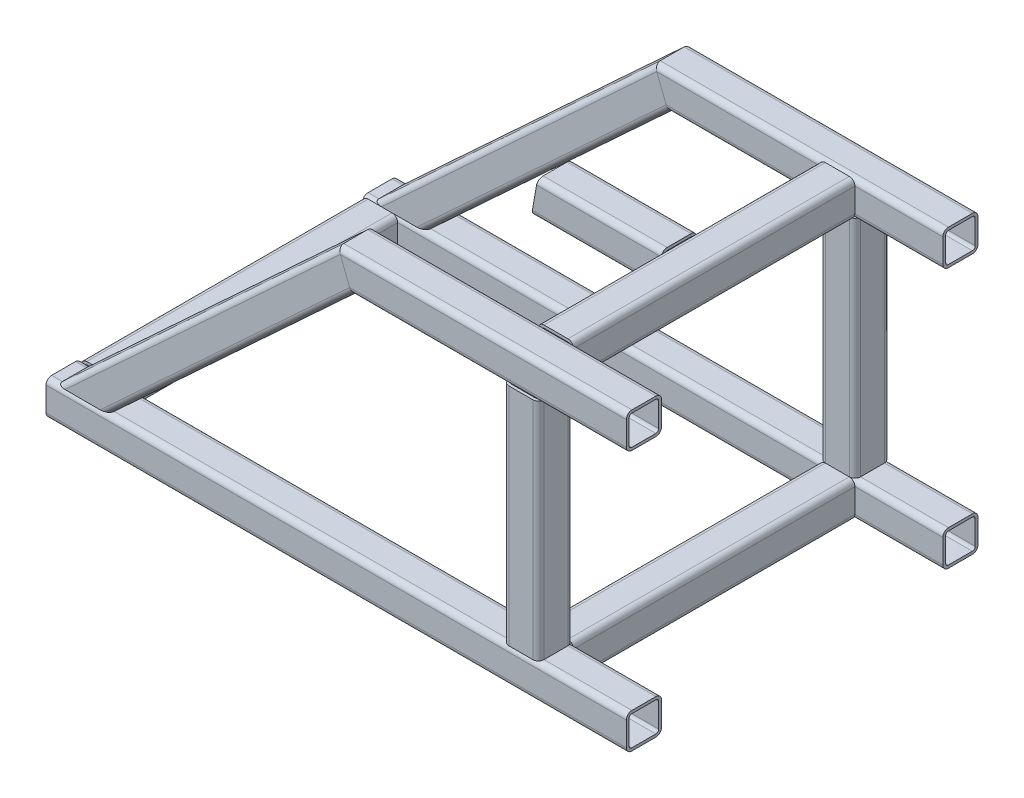
from build123d import *

# Parameters (mm, degrees)
GB_6728_1986_SQUARE_HOLLOW_SECTION_050_X_DEPTH = 400
GB_6728_1986_SQUARE_HOLLOW_SECTION_0_2_DEPTH   = 400
GB_6728_1986_SQUARE_HOLLOW_SECTION_0_3_DEPTH   = 825
GB_6728_1986_SQUARE_HOLLOW_SECTION_0_4_DEPTH   = 825
GB_6728_1986_SQUARE_HOLLOW_SECTION_0_5_DEPTH   = 211
GB_6728_1986_SQUARE_HOLLOW_SECTION_0_6_DEPTH   = 452
GB_6728_1986_SQUARE_HOLLOW_SECTION_0_8_DEPTH   = 372
GB_6728_1986_SQUARE_HOLLOW_SECTION_0_10_DEPTH  = 452
GB_6728_1986_SQUARE_HOLLOW_SECTION_0_13_DEPTH  = 372
GB_6728_1986_SQUARE_HOLLOW_SECTION_0_16_DEPTH  = 452
GB_6728_1986_SQUARE_HOLLOW_SECTION_0_19_DEPTH  = 544.885309033
GB_6728_1986_SQUARE_HOLLOW_SECTION_0_20_DEPTH  = 544.885309033
PART_RUN_ON_DEPTH                              = 409.789548
BODY_START                                     = 151.21090415
BODY_12_RUN_ON_DEPTH                           = 461.826729237
BODY_2_RUN_ON_DEPTH                            = 409.789548
BODY_11_RUN_ON_DEPTH                           = 461.826729237
CUT_EXTRUDE1_START                             = -50
CUT_EXTRUDE1_DEPTH                             = 50


with BuildPart() as part:
    # Sketch1 → Gb_6728-1986 square hollow section 050 X (new body)
    with BuildSketch(Plane(origin=(-250, 370, 450), x_dir=(0, 0, -1), z_dir=(1, 0, 0))):
        with BuildLine():
            Line((-17, -25), (17, -25))
            ThreePointArc((17, -25), (22.656854249, -22.656854249), (25, -17))
            Line((25, -17), (25, 17))
            ThreePointArc((25, 17), (22.656854249, 22.656854249), (17, 25))
            Line((17, 25), (-17, 25))
            ThreePointArc((-17, 25), (-22.656854249, 22.656854249), (-25, 17))
            Line((-25, 17), (-25, -17))
            ThreePointArc((-25, -17), (-22.656854249, -22.656854249), (-17, -25))
        make_face()
        with BuildLine():
            Line((-17, -21), (17, -21))
            ThreePointArc((17, -21), (19.828427125, -19.828427125), (21, -17))
            Line((21, -17), (21, 17))
            ThreePointArc((21, 17), (19.828427125, 19.828427125), (17, 21))
            Line((17, 21), (-17, 21))
            ThreePointArc((-17, 21), (-19.828427125, 19.828427125), (-21, 17))
            Line((-21, 17), (-21, -17))
            ThreePointArc((-21, -17), (-19.828427125, -19.828427125), (-17, -21))
        make_face(mode=Mode.SUBTRACT)
    extrude(amount=GB_6728_1986_SQUARE_HOLLOW_SECTION_050_X_DEPTH)

    # Sketch1 → part run on (add)
    with BuildSketch(Plane(origin=(-250, 370, 450), x_dir=(0, 0, -1), z_dir=(1, 0, 0))):
        with BuildLine():
            Line((-17, -25), (17, -25))
            ThreePointArc((17, -25), (22.656854249, -22.656854249), (25, -17))
            Line((25, -17), (25, 17))
            ThreePointArc((25, 17), (22.656854249, 22.656854249), (17, 25))
            Line((17, 25), (-17, 25))
            ThreePointArc((-17, 25), (-22.656854249, 22.656854249), (-25, 17))
            Line((-25, 17), (-25, -17))
            ThreePointArc((-25, -17), (-22.656854249, -22.656854249), (-17, -25))
        make_face()
        with BuildLine():
            Line((-17, -21), (17, -21))
            ThreePointArc((17, -21), (19.828427125, -19.828427125), (21, -17))
            Line((21, -17), (21, 17))
            ThreePointArc((21, 17), (19.828427125, 19.828427125), (17, 21))
            Line((17, 21), (-17, 21))
            ThreePointArc((-17, 21), (-19.828427125, 19.828427125), (-21, 17))
            Line((-21, 17), (-21, -17))
            ThreePointArc((-21, -17), (-19.828427125, -19.828427125), (-17, -21))
        make_face(mode=Mode.SUBTRACT)
    extrude(amount=-PART_RUN_ON_DEPTH)

    # Trim/Extend 3
    split(bisect_by=Plane(origin=(-250, 370, 450), x_dir=(-0.364623477, 0.931155046, 0), z_dir=(0.931155046, 0.364623477, 0)), keep=Keep.TOP)


with BuildPart() as body_2:
    # Sketch1 on segment 2 (carried to segment 2) → Gb_6728-1986 square hollow section 0 2 (new body)
    with BuildSketch(Plane(origin=(-250, 370, 0), x_dir=(0, 0, -1), z_dir=(1, 0, 0))):
        with BuildLine():
            Line((-17, -25), (17, -25))
            ThreePointArc((17, -25), (22.656854249, -22.656854249), (25, -17))
            Line((25, -17), (25, 17))
            ThreePointArc((25, 17), (22.656854249, 22.656854249), (17, 25))
            Line((17, 25), (-17, 25))
            ThreePointArc((-17, 25), (-22.656854249, 22.656854249), (-25, 17))
            Line((-25, 17), (-25, -17))
            ThreePointArc((-25, -17), (-22.656854249, -22.656854249), (-17, -25))
        make_face()
        with BuildLine():
            Line((-17, -21), (17, -21))
            ThreePointArc((17, -21), (19.828427125, -19.828427125), (21, -17))
            Line((21, -17), (21, 17))
            ThreePointArc((21, 17), (19.828427125, 19.828427125), (17, 21))
            Line((17, 21), (-17, 21))
            ThreePointArc((-17, 21), (-19.828427125, 19.828427125), (-21, 17))
            Line((-21, 17), (-21, -17))
            ThreePointArc((-21, -17), (-19.828427125, -19.828427125), (-17, -21))
        make_face(mode=Mode.SUBTRACT)
    extrude(amount=GB_6728_1986_SQUARE_HOLLOW_SECTION_0_2_DEPTH)

    # Sketch1 on segment 2 (carried to segment 2) → body 2 run on (add)
    with BuildSketch(Plane(origin=(-250, 370, 0), x_dir=(0, 0, -1), z_dir=(1, 0, 0))):
        with BuildLine():
            Line((-17, -25), (17, -25))
            ThreePointArc((17, -25), (22.656854249, -22.656854249), (25, -17))
            Line((25, -17), (25, 17))
            ThreePointArc((25, 17), (22.656854249, 22.656854249), (17, 25))
            Line((17, 25), (-17, 25))
            ThreePointArc((-17, 25), (-22.656854249, 22.656854249), (-25, 17))
            Line((-25, 17), (-25, -17))
            ThreePointArc((-25, -17), (-22.656854249, -22.656854249), (-17, -25))
        make_face()
        with BuildLine():
            Line((-17, -21), (17, -21))
            ThreePointArc((17, -21), (19.828427125, -19.828427125), (21, -17))
            Line((21, -17), (21, 17))
            ThreePointArc((21, 17), (19.828427125, 19.828427125), (17, 21))
            Line((17, 21), (-17, 21))
            ThreePointArc((-17, 21), (-19.828427125, 19.828427125), (-21, 17))
            Line((-21, 17), (-21, -17))
            ThreePointArc((-21, -17), (-19.828427125, -19.828427125), (-17, -21))
        make_face(mode=Mode.SUBTRACT)
    extrude(amount=-BODY_2_RUN_ON_DEPTH)

    # Trim/Extend 4
    split(bisect_by=Plane(origin=(-250, 370, 0), x_dir=(-0.364623477, 0.931155046, 0), z_dir=(0.931155046, 0.364623477, 0)), keep=Keep.TOP)


with BuildPart() as body_3:
    # Sketch1 on segment 3 (carried to segment 3) → Gb_6728-1986 square hollow section 0 3 (new body)
    with BuildSketch(Plane(origin=(-675, 0, 450), x_dir=(0, 0, -1), z_dir=(1, 0, 0))):
        with BuildLine():
            Line((-17, -25), (17, -25))
            ThreePointArc((17, -25), (22.656854249, -22.656854249), (25, -17))
            Line((25, -17), (25, 17))
            ThreePointArc((25, 17), (22.656854249, 22.656854249), (17, 25))
            Line((17, 25), (-17, 25))
            ThreePointArc((-17, 25), (-22.656854249, 22.656854249), (-25, 17))
            Line((-25, 17), (-25, -17))
            ThreePointArc((-25, -17), (-22.656854249, -22.656854249), (-17, -25))
        make_face()
        with BuildLine():
            Line((-17, -21), (17, -21))
            ThreePointArc((17, -21), (19.828427125, -19.828427125), (21, -17))
            Line((21, -17), (21, 17))
            ThreePointArc((21, 17), (19.828427125, 19.828427125), (17, 21))
            Line((17, 21), (-17, 21))
            ThreePointArc((-17, 21), (-19.828427125, 19.828427125), (-21, 17))
            Line((-21, 17), (-21, -17))
            ThreePointArc((-21, -17), (-19.828427125, -19.828427125), (-17, -21))
        make_face(mode=Mode.SUBTRACT)
    extrude(amount=GB_6728_1986_SQUARE_HOLLOW_SECTION_0_3_DEPTH)


with BuildPart() as body_4:
    # Sketch1 on segment 4 (carried to segment 4) → Gb_6728-1986 square hollow section 0 4 (new body)
    with BuildSketch(Plane(origin=(-675, 0, 0), x_dir=(0, 0, -1), z_dir=(1, 0, 0))):
        with BuildLine():
            Line((-17, -25), (17, -25))
            ThreePointArc((17, -25), (22.656854249, -22.656854249), (25, -17))
            Line((25, -17), (25, 17))
            ThreePointArc((25, 17), (22.656854249, 22.656854249), (17, 25))
            Line((17, 25), (-17, 25))
            ThreePointArc((-17, 25), (-22.656854249, 22.656854249), (-25, 17))
            Line((-25, 17), (-25, -17))
            ThreePointArc((-25, -17), (-22.656854249, -22.656854249), (-17, -25))
        make_face()
        with BuildLine():
            Line((-17, -21), (17, -21))
            ThreePointArc((17, -21), (19.828427125, -19.828427125), (21, -17))
            Line((21, -17), (21, 17))
            ThreePointArc((21, 17), (19.828427125, 19.828427125), (17, 21))
            Line((17, 21), (-17, 21))
            ThreePointArc((-17, 21), (-19.828427125, 19.828427125), (-21, 17))
            Line((-21, 17), (-21, -17))
            ThreePointArc((-21, -17), (-19.828427125, -19.828427125), (-17, -21))
        make_face(mode=Mode.SUBTRACT)
    extrude(amount=GB_6728_1986_SQUARE_HOLLOW_SECTION_0_4_DEPTH)


with BuildPart() as body_5:
    # Sketch1 on segment 5 (carried to segment 5) → Gb_6728-1986 square hollow section 0 5 (new body)
    with BuildSketch(Plane(origin=(-210, 370, 225), x_dir=(0, 0, -1), z_dir=(1, 0, 0))):
        with BuildLine():
            Line((-17, -25), (17, -25))
            ThreePointArc((17, -25), (22.656854249, -22.656854249), (25, -17))
            Line((25, -17), (25, 17))
            ThreePointArc((25, 17), (22.656854249, 22.656854249), (17, 25))
            Line((17, 25), (-17, 25))
            ThreePointArc((-17, 25), (-22.656854249, 22.656854249), (-25, 17))
            Line((-25, 17), (-25, -17))
            ThreePointArc((-25, -17), (-22.656854249, -22.656854249), (-17, -25))
        make_face()
        with BuildLine():
            Line((-17, -21), (17, -21))
            ThreePointArc((17, -21), (19.828427125, -19.828427125), (21, -17))
            Line((21, -17), (21, 17))
            ThreePointArc((21, 17), (19.828427125, 19.828427125), (17, 21))
            Line((17, 21), (-17, 21))
            ThreePointArc((-17, 21), (-19.828427125, 19.828427125), (-21, 17))
            Line((-21, 17), (-21, -17))
            ThreePointArc((-21, -17), (-19.828427125, -19.828427125), (-17, -21))
        make_face(mode=Mode.SUBTRACT)
    extrude(amount=GB_6728_1986_SQUARE_HOLLOW_SECTION_0_5_DEPTH)

    # Gb_6728-1986 square hollow section 0 5 e
    split(bisect_by=Plane(origin=(-25, 370, 225), x_dir=(0, -1, 0), z_dir=(-1, 0, 0)), keep=Keep.TOP)

    # Sketch3 → Cut-Extrude1 (cut)
    with BuildSketch(Plane(origin=(0, 0, 200), x_dir=(-1, 0, 0), z_dir=(0, 0, -1)).offset(CUT_EXTRUDE1_START)):
        Polygon((210, 345), (210, 395), (201.183650965, 395), align=None)
    extrude(amount=CUT_EXTRUDE1_DEPTH, mode=Mode.SUBTRACT)


with BuildPart() as body_6:
    # Sketch1 on segment 6 (carried to segment 6) → Gb_6728-1986 square hollow section 0 6 (new body)
    with BuildSketch(Plane(origin=(0, 370, -1), x_dir=(1, 0, 0), z_dir=(0, 0, 1))):
        with BuildLine():
            Line((-17, -25), (17, -25))
            ThreePointArc((17, -25), (22.656854249, -22.656854249), (25, -17))
            Line((25, -17), (25, 17))
            ThreePointArc((25, 17), (22.656854249, 22.656854249), (17, 25))
            Line((17, 25), (-17, 25))
            ThreePointArc((-17, 25), (-22.656854249, 22.656854249), (-25, 17))
            Line((-25, 17), (-25, -17))
            ThreePointArc((-25, -17), (-22.656854249, -22.656854249), (-17, -25))
        make_face()
        with BuildLine():
            Line((-17, -21), (17, -21))
            ThreePointArc((17, -21), (19.828427125, -19.828427125), (21, -17))
            Line((21, -17), (21, 17))
            ThreePointArc((21, 17), (19.828427125, 19.828427125), (17, 21))
            Line((17, 21), (-17, 21))
            ThreePointArc((-17, 21), (-19.828427125, 19.828427125), (-21, 17))
            Line((-21, 17), (-21, -17))
            ThreePointArc((-21, -17), (-19.828427125, -19.828427125), (-17, -21))
        make_face(mode=Mode.SUBTRACT)
    extrude(amount=GB_6728_1986_SQUARE_HOLLOW_SECTION_0_6_DEPTH)

    # Gb_6728-1986 square hollow section 0 6 e
    split(bisect_by=Plane(origin=(0, 370, 25), x_dir=(0, -1, 0), z_dir=(0, 0, 1)), keep=Keep.TOP)

    # Gb_6728-1986 square hollow section 0 7
    split(bisect_by=Plane(origin=(0, 370, 425), x_dir=(0, 1, 0), z_dir=(0, 0, -1)), keep=Keep.TOP)


with BuildPart() as body_7:
    # Sketch1 on segment 7 (carried to segment 7) → Gb_6728-1986 square hollow section 0 8 (new body)
    with BuildSketch(Plane(origin=(0, -1, 450), x_dir=(0, 0, -1), z_dir=(0, 1, 0))):
        with BuildLine():
            Line((-17, -25), (17, -25))
            ThreePointArc((17, -25), (22.656854249, -22.656854249), (25, -17))
            Line((25, -17), (25, 17))
            ThreePointArc((25, 17), (22.656854249, 22.656854249), (17, 25))
            Line((17, 25), (-17, 25))
            ThreePointArc((-17, 25), (-22.656854249, 22.656854249), (-25, 17))
            Line((-25, 17), (-25, -17))
            ThreePointArc((-25, -17), (-22.656854249, -22.656854249), (-17, -25))
        make_face()
        with BuildLine():
            Line((-17, -21), (17, -21))
            ThreePointArc((17, -21), (19.828427125, -19.828427125), (21, -17))
            Line((21, -17), (21, 17))
            ThreePointArc((21, 17), (19.828427125, 19.828427125), (17, 21))
            Line((17, 21), (-17, 21))
            ThreePointArc((-17, 21), (-19.828427125, 19.828427125), (-21, 17))
            Line((-21, 17), (-21, -17))
            ThreePointArc((-21, -17), (-19.828427125, -19.828427125), (-17, -21))
        make_face(mode=Mode.SUBTRACT)
    extrude(amount=GB_6728_1986_SQUARE_HOLLOW_SECTION_0_8_DEPTH)

    # Gb_6728-1986 square hollow section 0 8 e
    split(bisect_by=Plane(origin=(0, 25, 450), x_dir=(-1, 0, 0), z_dir=(0, 1, 0)), keep=Keep.TOP)

    # Gb_6728-1986 square hollow section 0 9
    split(bisect_by=Plane(origin=(0, 345, 450), x_dir=(1, 0, 0), z_dir=(0, -1, 0)), keep=Keep.TOP)


with BuildPart() as body_8:
    # Sketch1 on segment 8 (carried to segment 8) → Gb_6728-1986 square hollow section 0 10 (new body)
    with BuildSketch(Plane.XY.offset(-1)):
        with BuildLine():
            Line((-17, -25), (17, -25))
            ThreePointArc((17, -25), (22.656854249, -22.656854249), (25, -17))
            Line((25, -17), (25, 17))
            ThreePointArc((25, 17), (22.656854249, 22.656854249), (17, 25))
            Line((17, 25), (-17, 25))
            ThreePointArc((-17, 25), (-22.656854249, 22.656854249), (-25, 17))
            Line((-25, 17), (-25, -17))
            ThreePointArc((-25, -17), (-22.656854249, -22.656854249), (-17, -25))
        make_face()
        with BuildLine():
            Line((-17, -21), (17, -21))
            ThreePointArc((17, -21), (19.828427125, -19.828427125), (21, -17))
            Line((21, -17), (21, 17))
            ThreePointArc((21, 17), (19.828427125, 19.828427125), (17, 21))
            Line((17, 21), (-17, 21))
            ThreePointArc((-17, 21), (-19.828427125, 19.828427125), (-21, 17))
            Line((-21, 17), (-21, -17))
            ThreePointArc((-21, -17), (-19.828427125, -19.828427125), (-17, -21))
        make_face(mode=Mode.SUBTRACT)
    extrude(amount=GB_6728_1986_SQUARE_HOLLOW_SECTION_0_10_DEPTH)

    # Gb_6728-1986 square hollow section 0 11
    split(bisect_by=Plane(origin=(0, 0, 25), x_dir=(0, -1, 0), z_dir=(0, 0, 1)), keep=Keep.TOP)

    # Gb_6728-1986 square hollow section 0 12
    split(bisect_by=Plane.YX.offset(-425), keep=Keep.TOP)


with BuildPart() as body_9:
    # Sketch1 on segment 9 (carried to segment 9) → Gb_6728-1986 square hollow section 0 13 (new body)
    with BuildSketch(Plane(origin=(0, -1, 0), x_dir=(0, 0, -1), z_dir=(0, 1, 0))):
        with BuildLine():
            Line((-17, -25), (17, -25))
            ThreePointArc((17, -25), (22.656854249, -22.656854249), (25, -17))
            Line((25, -17), (25, 17))
            ThreePointArc((25, 17), (22.656854249, 22.656854249), (17, 25))
            Line((17, 25), (-17, 25))
            ThreePointArc((-17, 25), (-22.656854249, 22.656854249), (-25, 17))
            Line((-25, 17), (-25, -17))
            ThreePointArc((-25, -17), (-22.656854249, -22.656854249), (-17, -25))
        make_face()
        with BuildLine():
            Line((-17, -21), (17, -21))
            ThreePointArc((17, -21), (19.828427125, -19.828427125), (21, -17))
            Line((21, -17), (21, 17))
            ThreePointArc((21, 17), (19.828427125, 19.828427125), (17, 21))
            Line((17, 21), (-17, 21))
            ThreePointArc((-17, 21), (-19.828427125, 19.828427125), (-21, 17))
            Line((-21, 17), (-21, -17))
            ThreePointArc((-21, -17), (-19.828427125, -19.828427125), (-17, -21))
        make_face(mode=Mode.SUBTRACT)
    extrude(amount=GB_6728_1986_SQUARE_HOLLOW_SECTION_0_13_DEPTH)

    # Gb_6728-1986 square hollow section 0 14
    split(bisect_by=Plane(origin=(0, 25, 0), x_dir=(-1, 0, 0), z_dir=(0, 1, 0)), keep=Keep.TOP)

    # Gb_6728-1986 square hollow section 0 15
    split(bisect_by=Plane.XZ.offset(-345), keep=Keep.TOP)


with BuildPart() as body_10:
    # Sketch1 on segment 10 (carried to segment 10) → Gb_6728-1986 square hollow section 0 16 (new body)
    with BuildSketch(Plane(origin=(-650, 0, -1), x_dir=(1, 0, 0), z_dir=(0, 0, 1))):
        with BuildLine():
            Line((-17, -25), (17, -25))
            ThreePointArc((17, -25), (22.656854249, -22.656854249), (25, -17))
            Line((25, -17), (25, 17))
            ThreePointArc((25, 17), (22.656854249, 22.656854249), (17, 25))
            Line((17, 25), (-17, 25))
            ThreePointArc((-17, 25), (-22.656854249, 22.656854249), (-25, 17))
            Line((-25, 17), (-25, -17))
            ThreePointArc((-25, -17), (-22.656854249, -22.656854249), (-17, -25))
        make_face()
        with BuildLine():
            Line((-17, -21), (17, -21))
            ThreePointArc((17, -21), (19.828427125, -19.828427125), (21, -17))
            Line((21, -17), (21, 17))
            ThreePointArc((21, 17), (19.828427125, 19.828427125), (17, 21))
            Line((17, 21), (-17, 21))
            ThreePointArc((-17, 21), (-19.828427125, 19.828427125), (-21, 17))
            Line((-21, 17), (-21, -17))
            ThreePointArc((-21, -17), (-19.828427125, -19.828427125), (-17, -21))
        make_face(mode=Mode.SUBTRACT)
    extrude(amount=GB_6728_1986_SQUARE_HOLLOW_SECTION_0_16_DEPTH)

    # Gb_6728-1986 square hollow section 0 17
    split(bisect_by=Plane(origin=(-650, 0, 25), x_dir=(0, -1, 0), z_dir=(0, 0, 1)), keep=Keep.TOP)

    # Gb_6728-1986 square hollow section 0 18
    split(bisect_by=Plane(origin=(-650, 0, 425), x_dir=(0, 1, 0), z_dir=(0, 0, -1)), keep=Keep.TOP)


with BuildPart() as body_11:
    # Sketch11 → Gb_6728-1986 square hollow section 0 19 (new body)
    with BuildSketch(Plane(origin=(-250, 370, 0), x_dir=(0.6790419816174272, -0.7340994395864077, 0), z_dir=(-0.7340994395864077, -0.6790419816174272, 0))):
        with BuildLine():
            Line((-17, -25), (17, -25))
            ThreePointArc((17, -25), (22.656854249, -22.656854249), (25, -17))
            Line((25, -17), (25, 17))
            ThreePointArc((25, 17), (22.656854249, 22.656854249), (17, 25))
            Line((17, 25), (-17, 25))
            ThreePointArc((-17, 25), (-22.656854249, 22.656854249), (-25, 17))
            Line((-25, 17), (-25, -17))
            ThreePointArc((-25, -17), (-22.656854249, -22.656854249), (-17, -25))
        make_face()
        with BuildLine():
            Line((-17, -21), (17, -21))
            ThreePointArc((17, -21), (19.828427125, -19.828427125), (21, -17))
            Line((21, -17), (21, 17))
            ThreePointArc((21, 17), (19.828427125, 19.828427125), (17, 21))
            Line((17, 21), (-17, 21))
            ThreePointArc((-17, 21), (-19.828427125, 19.828427125), (-21, 17))
            Line((-21, 17), (-21, -17))
            ThreePointArc((-21, -17), (-19.828427125, -19.828427125), (-17, -21))
        make_face(mode=Mode.SUBTRACT)
    extrude(amount=GB_6728_1986_SQUARE_HOLLOW_SECTION_0_19_DEPTH)

    # Trim/Extend 2
    split(bisect_by=Plane(origin=(-50, 345, 0), x_dir=(1, 0, 0), z_dir=(0, -1, 0)), keep=Keep.TOP)

    # Trim_Extend 2 5
    split(bisect_by=Plane(origin=(-262.5, 25, 0), x_dir=(-1, 0, 0), z_dir=(0, 1, 0)), keep=Keep.TOP)

    # body 11 cut square before the run-on
    split(bisect_by=Plane(origin=(-361.003840059, 267.321447946, 0), x_dir=(0.679041982, -0.73409944, 0), z_dir=(-0.73409944, -0.679041982, 0)), keep=Keep.TOP)

    # Sketch11 → body 11 run on (add)
    with BuildSketch(Plane(origin=(-250, 370, 0), x_dir=(0.6790419816174272, -0.7340994395864077, 0), z_dir=(-0.7340994395864077, -0.6790419816174272, 0)).offset(BODY_START)):
        with BuildLine():
            Line((-17, -25), (17, -25))
            ThreePointArc((17, -25), (22.656854249, -22.656854249), (25, -17))
            Line((25, -17), (25, 17))
            ThreePointArc((25, 17), (22.656854249, 22.656854249), (17, 25))
            Line((17, 25), (-17, 25))
            ThreePointArc((-17, 25), (-22.656854249, 22.656854249), (-25, 17))
            Line((-25, 17), (-25, -17))
            ThreePointArc((-25, -17), (-22.656854249, -22.656854249), (-17, -25))
        make_face()
        with BuildLine():
            Line((-17, -21), (17, -21))
            ThreePointArc((17, -21), (19.828427125, -19.828427125), (21, -17))
            Line((21, -17), (21, 17))
            ThreePointArc((21, 17), (19.828427125, 19.828427125), (17, 21))
            Line((17, 21), (-17, 21))
            ThreePointArc((-17, 21), (-19.828427125, 19.828427125), (-21, 17))
            Line((-21, 17), (-21, -17))
            ThreePointArc((-21, -17), (-19.828427125, -19.828427125), (-17, -21))
        make_face(mode=Mode.SUBTRACT)
    extrude(amount=-BODY_11_RUN_ON_DEPTH)

    # Trim/Extend 4
    split(bisect_by=Plane(origin=(-250, 370, 0), x_dir=(0.364623477, -0.931155046, 0), z_dir=(-0.931155046, -0.364623477, 0)), keep=Keep.TOP)


with BuildPart() as body_12:
    # Sketch11 on segment 2 (carried to segment 2) → Gb_6728-1986 square hollow section 0 20 (new body)
    with BuildSketch(Plane(origin=(-250, 370, 450), x_dir=(0.679041982, -0.73409944, 0), z_dir=(-0.73409944, -0.679041982, 0))):
        with BuildLine():
            Line((-17, -25), (17, -25))
            ThreePointArc((17, -25), (22.656854249, -22.656854249), (25, -17))
            Line((25, -17), (25, 17))
            ThreePointArc((25, 17), (22.656854249, 22.656854249), (17, 25))
            Line((17, 25), (-17, 25))
            ThreePointArc((-17, 25), (-22.656854249, 22.656854249), (-25, 17))
            Line((-25, 17), (-25, -17))
            ThreePointArc((-25, -17), (-22.656854249, -22.656854249), (-17, -25))
        make_face()
        with BuildLine():
            Line((-17, -21), (17, -21))
            ThreePointArc((17, -21), (19.828427125, -19.828427125), (21, -17))
            Line((21, -17), (21, 17))
            ThreePointArc((21, 17), (19.828427125, 19.828427125), (17, 21))
            Line((17, 21), (-17, 21))
            ThreePointArc((-17, 21), (-19.828427125, 19.828427125), (-21, 17))
            Line((-21, 17), (-21, -17))
            ThreePointArc((-21, -17), (-19.828427125, -19.828427125), (-17, -21))
        make_face(mode=Mode.SUBTRACT)
    extrude(amount=GB_6728_1986_SQUARE_HOLLOW_SECTION_0_20_DEPTH)

    # Trim/Extend 2
    split(bisect_by=Plane(origin=(-50, 345, 0), x_dir=(1, 0, 0), z_dir=(0, -1, 0)), keep=Keep.TOP)

    # Trim_Extend 2 5
    split(bisect_by=Plane(origin=(-262.5, 25, 0), x_dir=(-1, 0, 0), z_dir=(0, 1, 0)), keep=Keep.TOP)

    # body 12 cut square before the run-on
    split(bisect_by=Plane(origin=(-361.003840059, 267.321447946, 450), x_dir=(0.679041982, -0.73409944, 0), z_dir=(-0.73409944, -0.679041982, 0)), keep=Keep.TOP)

    # Sketch11 on segment 2 (carried to segment 2) → body 12 run on (add)
    with BuildSketch(Plane(origin=(-250, 370, 450), x_dir=(0.679041982, -0.73409944, 0), z_dir=(-0.73409944, -0.679041982, 0)).offset(BODY_START)):
        with BuildLine():
            Line((-17, -25), (17, -25))
            ThreePointArc((17, -25), (22.656854249, -22.656854249), (25, -17))
            Line((25, -17), (25, 17))
            ThreePointArc((25, 17), (22.656854249, 22.656854249), (17, 25))
            Line((17, 25), (-17, 25))
            ThreePointArc((-17, 25), (-22.656854249, 22.656854249), (-25, 17))
            Line((-25, 17), (-25, -17))
            ThreePointArc((-25, -17), (-22.656854249, -22.656854249), (-17, -25))
        make_face()
        with BuildLine():
            Line((-17, -21), (17, -21))
            ThreePointArc((17, -21), (19.828427125, -19.828427125), (21, -17))
            Line((21, -17), (21, 17))
            ThreePointArc((21, 17), (19.828427125, 19.828427125), (17, 21))
            Line((17, 21), (-17, 21))
            ThreePointArc((-17, 21), (-19.828427125, 19.828427125), (-21, 17))
            Line((-21, 17), (-21, -17))
            ThreePointArc((-21, -17), (-19.828427125, -19.828427125), (-17, -21))
        make_face(mode=Mode.SUBTRACT)
    extrude(amount=-BODY_12_RUN_ON_DEPTH)

    # Trim/Extend 3
    split(bisect_by=Plane(origin=(-250, 370, 450), x_dir=(0.364623477, -0.931155046, 0), z_dir=(-0.931155046, -0.364623477, 0)), keep=Keep.TOP)


solid = Compound([part.part, body_2.part, body_3.part, body_4.part, body_5.part, body_6.part, body_7.part, body_8.part, body_9.part, body_10.part, body_11.part, body_12.part])
